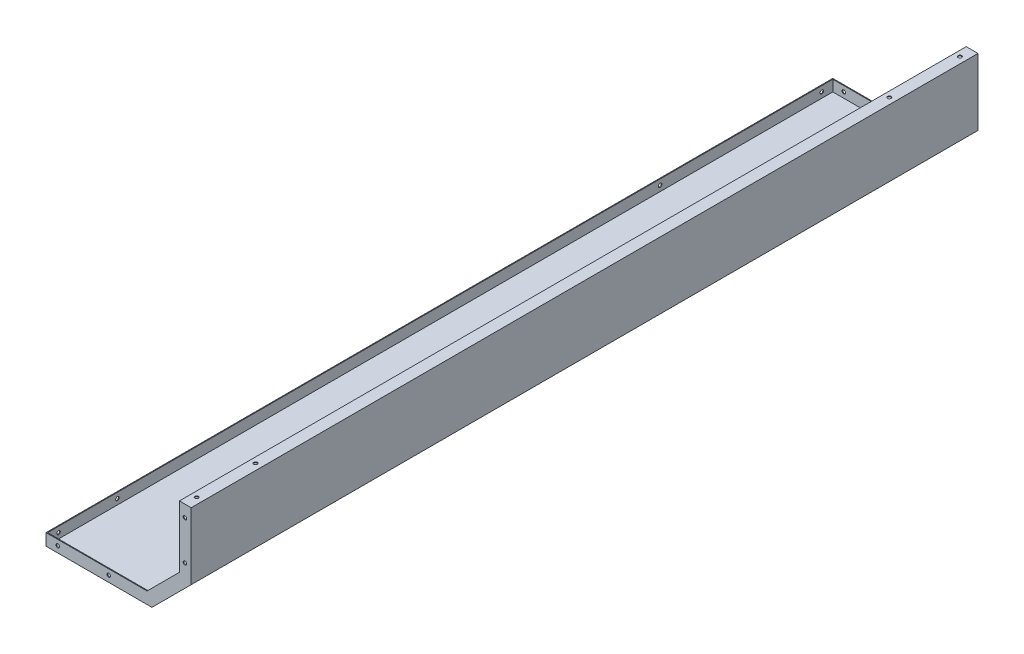
SolidWorks part; units mm, degrees
ref_plane "前视基准面" through (0, 0, 0) normal (0, 0, 1) x (1, 0, 0)
ref_plane "上视基准面" through (0, 0, 0) normal (0, 1, 0) x (1, 0, 0)
ref_plane "右视基准面" through (0, 0, 0) normal (1, 0, 0) x (0, 0, -1)
sketch "草图1" plane through (0, 0, 0) normal (0, 0, 1) x (1, 0, 0)
  line L0 (0, 0) -> (270, 0)
  line L1 (370, 100) -> (370, 270)
  line L2 (270, 0) -> (370, 100)
  point P1 (370, 0)
  dimension "D1" = 370
  dimension "D2" = 270
extrude "拉伸-薄壁1" add sketch "草图1" along normal blind 2005 thin thin type one direction reverse wall 2
sketch "草图4" plane through (368, 0, 0) normal (-1, 0, 0) x (0, 0, 1)
  line L0 (0, 100.8284) -> (0, 270)
  line L1 (0, 270) -> (2005, 270)
  line L2 (2005, 270) -> (2005, 100.8284)
  line L3 (2, 100.8284) -> (2, 268)
  line L4 (2, 268) -> (2003, 268)
  line L5 (2003, 268) -> (2003, 100.8284)
  line L6 (2003, 100.8284) -> (2005, 100.8284)
  line L7 (0, 100.8284) -> (2, 100.8284)
  dimension "D1" = 2
extrude "凸台-拉伸1" add sketch "草图4" along normal blind 28
sketch "草图5" plane through (133.5858, -133.5858, 0) normal (-0.7071, 0.7071, 0) x (0, 0, 1)
  line L0 (0, 331.5118) -> (0, 191.7473)
  line L1 (2005, 331.5118) -> (2005, 191.7473)
  line L2 (2003, 331.5118) -> (2003, 191.7473)
  line L3 (2, 331.5118) -> (2, 191.7473)
  line L4 (0, 331.5118) -> (2, 331.5118)
  line L5 (0, 191.7473) -> (2, 191.7473)
  line L6 (2003, 331.5118) -> (2005, 331.5118)
  line L7 (2003, 191.7473) -> (2005, 191.7473)
  dimension "D1" = 2
  dimension "D2" = 2
extrude "凸台-拉伸2" add sketch "草图5" along normal blind 28
sketch "草图6" plane through (0, 2, 0) normal (0, 1, 0) x (1, 0, 0)
  line L1 (0, 0) -> (269.1716, 0)
  line L2 (0, 0) -> (0, -2)
  line L3 (0, -2) -> (269.1716, -2)
  line L4 (269.1716, 0) -> (269.1716, -2)
  line L5 (0, -2005) -> (269.1716, -2005)
  line L6 (0, -2005) -> (0, -2003)
  line L7 (0, -2003) -> (269.1716, -2003)
  line L8 (269.1716, -2005) -> (269.1716, -2003)
extrude "凸台-拉伸3" add sketch "草图6" along normal blind 28
sketch "草图7" plane through (0, 2, 0) normal (0, 1, 0) x (1, 0, 0)
  line L0 (0, -2005) -> (257.5736, -2005) construction
  line L1 (0, 0) -> (2, 0)
  line L2 (0, 0) -> (0, -2005)
  line L3 (0, -2005) -> (2, -2005)
  line L4 (2, 0) -> (2, -2005)
  dimension "D1" = 2
extrude "凸台-拉伸4" add sketch "草图7" along normal blind 28
sketch "草图8" plane through (0, 0, 2003) normal (0, 0, -1) x (-1, 0, 0)
  line L0 (-354, 268) -> (-354, 101.2703) construction
  line L1 (-340, 268) -> (-368, 268) construction
  line L5 (-2, 16) -> (-237.543, 16) construction
  line L7 (-2, 2) -> (-2, 30) construction
  line L8 (-340, 270) -> (-370, 270) construction
  line L9 (0, 0) -> (0, 30) construction
  circle A0 centre (-354, 240) radius 4.5
  circle A1 centre (-30, 16) radius 4.5
  circle A2 centre (-354, 140) radius 4.5
  circle A3 centre (-160, 16) radius 4.5
  dimension "D1" = 9
  dimension "D2" = 9
  dimension "D3" = 9
  dimension "D4" = 9
  dimension "D5" = 30
  dimension "D6" = 30
  dimension "D7" = 130
  dimension "D8" = 100
extrude "切除-拉伸1" cut sketch "草图8" against normal blind 10 and the other way blind 10
sketch "草图9" plane through (0, 268, 0) normal (0, -1, 0) x (1, 0, 0)
  line L0 (354, 2003) -> (354, 1870.0821) construction
  line L1 (340, 2003) -> (368, 2003) construction
  line L2 (340, 2005) -> (370, 2005) construction
  circle A0 centre (354, 1975) radius 4.5
  circle A1 centre (354, 1825) radius 4.5
  dimension "D1" = 9
  dimension "D2" = 9
  dimension "D3" = 30
  dimension "D4" = 150
extrude "切除-拉伸2" cut sketch "草图9" against normal blind 10
sketch "草图10" plane through (2, 0, 0) normal (1, 0, 0) x (0, 0, -1)
  line L0 (-2003, 16) -> (-1811.8227, 16) construction
  line L1 (-2003, 30) -> (-2003, 2) construction
  line L2 (-2005, 0) -> (-2005, 30) construction
  circle A0 centre (-1975, 16) radius 4.5
  circle A1 centre (-1825, 16) radius 4.5
  dimension "D1" = 9
  dimension "D2" = 9
  dimension "D3" = 30
  dimension "D4" = 150
extrude "切除-拉伸3" cut sketch "草图10" against normal blind 76
sketch "草图11" plane through (0, 268, 0) normal (0, -1, 0) x (1, 0, 0)
  line L0 (354, 2) -> (354, 212.6561) construction
  line L1 (340, 2) -> (368, 2) construction
  line L2 (340, 0) -> (370, 0) construction
  circle A0 centre (354, 30) radius 4.5
  circle A1 centre (354, 210) radius 4.5
  dimension "D1" = 9
  dimension "D2" = 9
  dimension "D3" = 30
  dimension "D4" = 180
extrude "切除-拉伸4" cut sketch "草图11" against normal blind 63
sketch "草图12" plane through (2, 0, 0) normal (1, 0, 0) x (0, 0, -1)
  line L0 (-2, 16) -> (-391.141, 16) construction
  line L1 (-2, 2) -> (-2, 30) construction
  line L2 (0, 0) -> (0, 30) construction
  circle A0 centre (-30, 16) radius 4.5
  circle A1 centre (-442, 16) radius 4.5
  dimension "D1" = 9
  dimension "D2" = 9
  dimension "D3" = 412
  dimension "D4" = 30
extrude "切除-拉伸5" cut sketch "草图12" against normal blind 10
sketch "草图13" plane through (0, 0, 0) normal (0, 0, -1) x (-1, 0, 0)
  line L14 (-340, 270) -> (-370, 270) construction
  line L15 (0, 0) -> (0, 30) construction
  line L17 (-354, 270) -> (-354, 106.6274)
  line L18 (-354, 106.6274) -> (-263.3726, 16)
  line L19 (-263.3726, 16) -> (0, 16)
  line L20 (-354, 270) -> (-354, 106.6274) construction
  line L21 (-354, 106.6274) -> (-263.3726, 16) construction
  line L22 (-263.3726, 16) -> (0, 16) construction
  circle A0 centre (-30, 16) radius 4.5
  circle A1 centre (-354, 240) radius 4.5
  circle A2 centre (-308.6863, 61.3137) radius 4.5
  dimension "D2" = 9
  dimension "D3" = 9
  dimension "D4" = 9
  dimension "D5" = 30
  dimension "D6" = 30
  dimension "D1" = 14
extrude "切除-拉伸6" cut sketch "草图13" against normal blind 10
